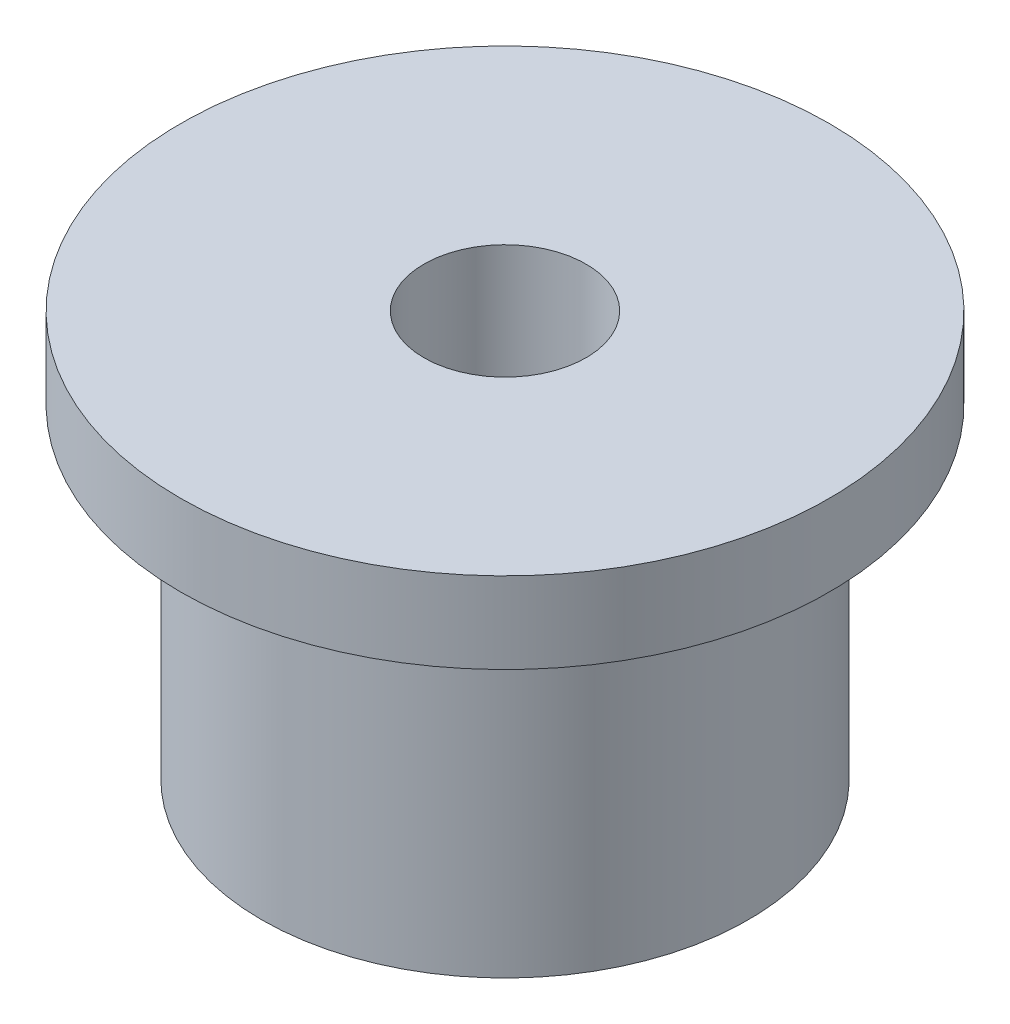
from build123d import *


with BuildPart() as part:
    # Sketch1 → Revolve1 (revolve)
    with BuildSketch(Plane.XY, mode=Mode.PRIVATE) as revolve1_sk:
        Polygon((-25, 0), (-100, 0), (-100, -25), (-75, -25), (-75, -125), (-25, -125), align=None)
    revolve(revolve1_sk.sketch.rotate(Axis((0, 71.088290965, 0), (0, -1, 0)), 270), axis=Axis((0, 71.088290965, 0), (0, -1, 0)))


solid = part.part
